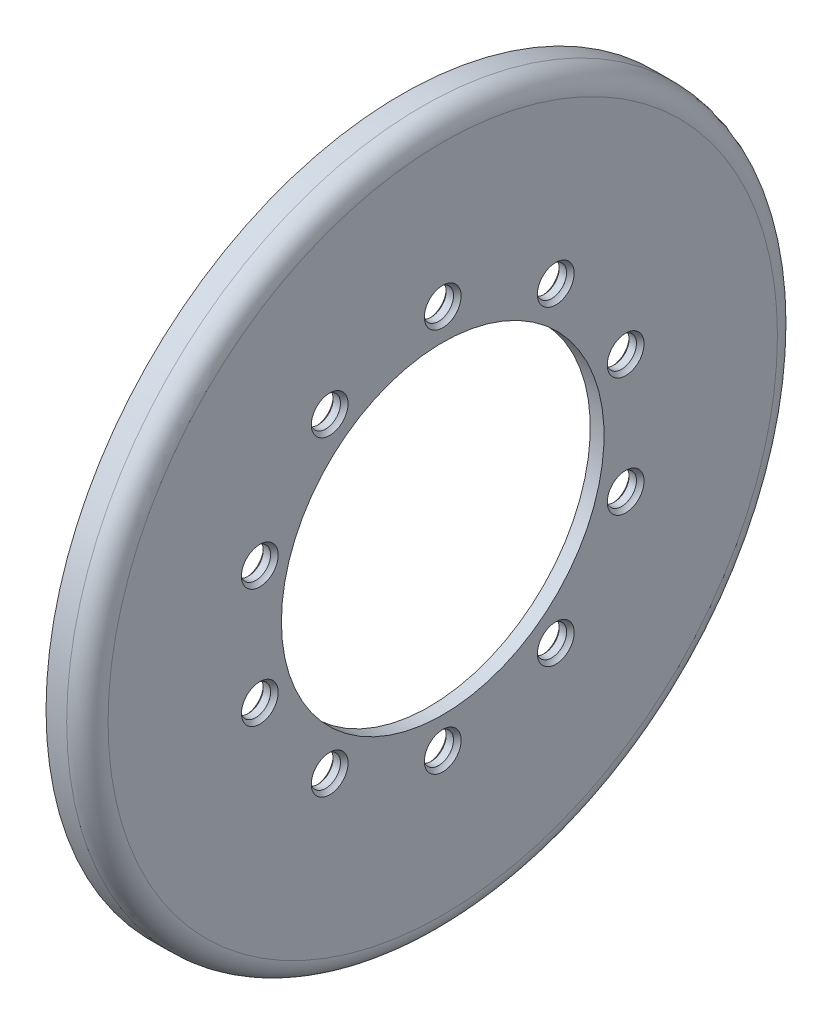
SolidWorks part; units mm, degrees
material "普通碳钢"
ref_plane "前视" through (0, 0, 0) normal (0, 0, 1) x (1, 0, 0)
ref_plane "上视" through (0, 0, 0) normal (0, 1, 0) x (1, 0, 0)
ref_plane "右视" through (0, 0, 0) normal (1, 0, 0) x (0, 0, -1)
sketch "草图1" plane through (0, 0, 0) normal (0, 0, 1) x (1, 0, 0)
  line L0 (-295.4, 0) -> (260.4, 0) construction
  line L1 (0, 207.55) -> (0, -191.45) construction
  line L2 (0, 309.5) -> (36, 309.5)
  line L3 (36, 309.5) -> (36, 140.5)
  line L4 (36, 140.5) -> (24, 140.5)
  line L5 (22, 217.5) -> (22, 295.5)
  line L6 (22, 295.5) -> (0, 295.5)
  line L7 (0, 295.5) -> (0, 309.5)
  line L8 (22, 217.5) -> (24, 217.5)
  line L9 (24, 217.5) -> (24, 140.5)
  dimension "D1" = 14
  dimension "D2" = 14
  dimension "D3" = 22
  dimension "D4" = 2
  dimension "D5" = 309.5
  dimension "D6" = 281
  dimension "D7" = 435
revolve "旋转1" add sketch "草图1" angle 360 about L0
fillet "圆角1" radius 18 1 edges at (36, 0, 309.5)
fillet "圆角2" radius 4 1 edges at (22, 0, 295.5)
sketch "草图2" plane through (36, 0, 0) normal (1, 0, 0) x (0, 0, -1)
  circle A0 centre (0, 167.5) radius 13
  dimension "D1" = 26
  dimension "D2" = 167.5
extrude "切除-拉伸1" cut sketch "草图2" against normal through all
chamfer "倒角1" distance 2 angle 45 1 edges at (24, 167.5, -13)
sketch "草图3" plane through (0, 0, 0) normal (0, 0, 1) x (1, 0, 0)
  line L0 (26, 167.5) -> (36, 167.5) construction
  line L1 (32.3981, 180.5081) -> (32.3981, 167.5)
  line L2 (32.3981, 167.5) -> (65.247, 167.5)
  line L4 (36, -291.5) -> (36, 291.5) construction
  arc A0 (65.247, 167.5) -> (32.3981, 180.5081) centre (46.247, 167.5) ccw
  point P4 (32.3981, 180.5081)
  point P8 (36, 183.5)
  point P9 (36, 151.5)
  dimension "D1" = 38
  dimension "D2" = 16
  dimension "D3" = 16
revolve "切除-旋转1" cut sketch "草图3" angle 360 about axis through (0, 167.5, 0) along (1, 0, 0)
pattern_circular "阵列(圆周)1" count 10 over 360 about axis through (0, 0, 0) along (1, 0, 0) of "切除-旋转1", "切除-拉伸1", "倒角1"
